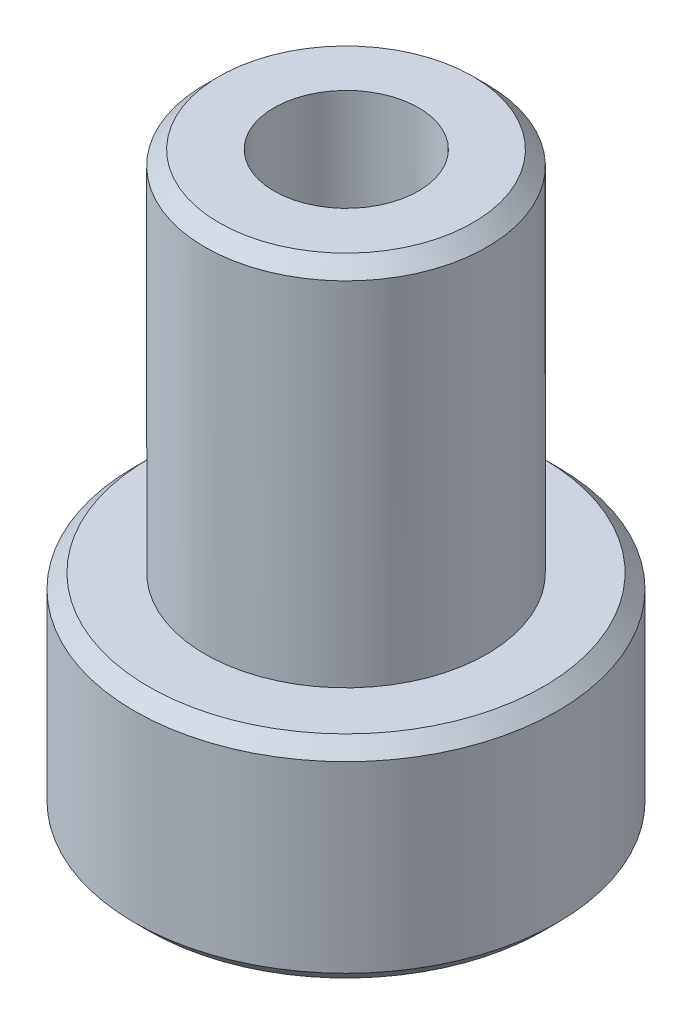
from build123d import *

# Parameters (mm, degrees)
SKETCH1_R               = 2
BOSS_EXTRUDE1_DEPTH     = 8.2
M2_5_TAPPED_HOLE1_D     = 2.05
M2_5_TAPPED_HOLE1_DEPTH = 6.35
M2_5_TAPPED_HOLE1_TIP   = 0.615882135
SKETCH8_R               = 3
BOSS_EXTRUDE2_DEPTH     = 3
CHAMFER1_SIZE           = 0.2
CHAMFER2_SIZE           = 0.2


with BuildPart() as part:
    # Sketch1 → Boss-Extrude1 (new body)
    with BuildSketch(Plane(origin=(0, 0, 0), x_dir=(1, 0, 0), z_dir=(0, 1, 0))):
        with Locations(Location((0, 0, 0), (0, 0, 270))):
            Circle(SKETCH1_R)
    extrude(amount=BOSS_EXTRUDE1_DEPTH)

    # M2.5 Tapped Hole1
    with Locations(Plane(origin=(0, 8.2, 0), x_dir=(1, 0, 0), z_dir=(0, 1, 0))):
        with Locations((0, 0.004175621)):
            Hole(M2_5_TAPPED_HOLE1_D / 2, depth=M2_5_TAPPED_HOLE1_DEPTH)
            with Locations((0, 0, -(M2_5_TAPPED_HOLE1_DEPTH + M2_5_TAPPED_HOLE1_TIP / 2))):  # 118° drill point
                Cone(0, M2_5_TAPPED_HOLE1_D / 2, M2_5_TAPPED_HOLE1_TIP, mode=Mode.SUBTRACT)

    # Sketch8 → Boss-Extrude2 (add)
    with BuildSketch(Plane.XZ):
        with Locations(Location((0, 0, 0), (0, 0, 270))):
            Circle(SKETCH8_R)
    extrude(amount=-BOSS_EXTRUDE2_DEPTH)

    # Chamfer1
    chamfer1_edges = [part.edges().sort_by_distance(p)[0] for p in [
        (0, 8.2, -2),
    ]]
    chamfer(chamfer1_edges, length=CHAMFER1_SIZE)

    # Chamfer2
    chamfer2_edges = [part.edges().sort_by_distance(p)[0] for p in [
        (0, 0, 3),
        (0, 3, 3),
    ]]
    chamfer(chamfer2_edges, length=CHAMFER2_SIZE)


solid = part.part
